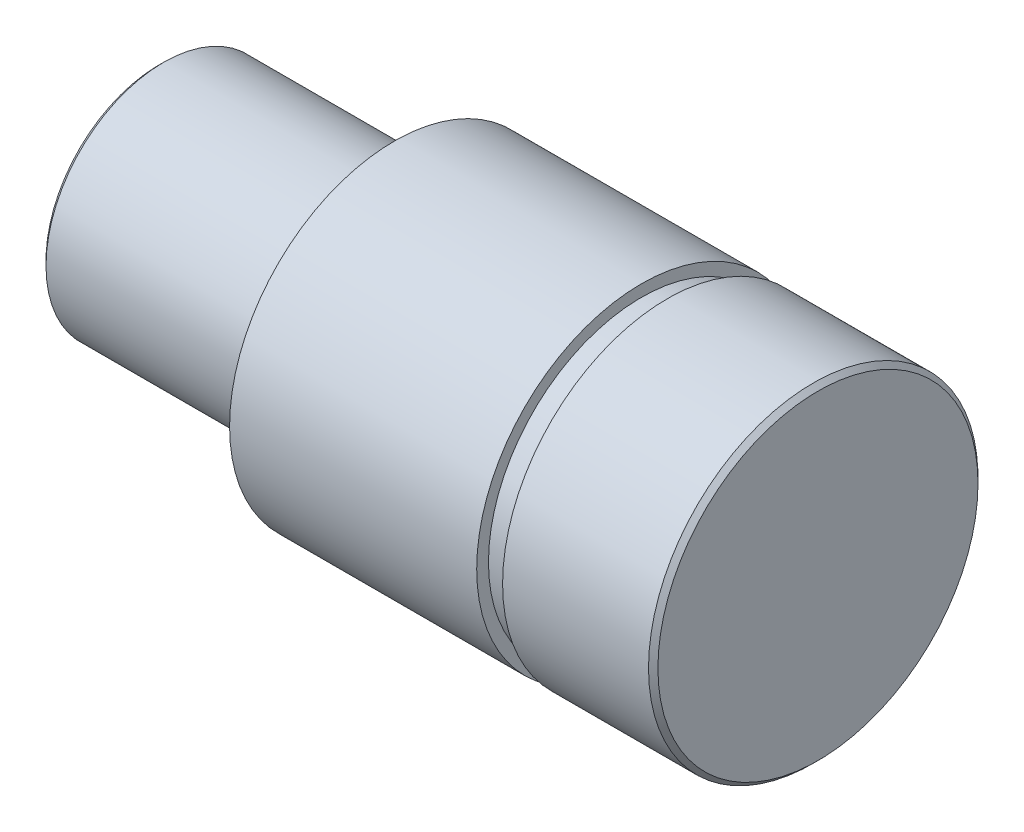
SolidWorks part; units mm, degrees
ref_plane "Front Plane" through (0, 0, 0) normal (0, 0, 1) x (1, 0, 0)
ref_plane "Top Plane" through (0, 0, 0) normal (0, 1, 0) x (1, 0, 0)
ref_plane "Right Plane" through (0, 0, 0) normal (1, 0, 0) x (0, 0, -1)
sketch "Sketch1" plane through (0, 0, 0) normal (0, 0, 1) x (1, 0, 0)
  line L0 (0, 0) -> (40.5225, 0) construction
  line L1 (0, 0) -> (0, 5)
  line L2 (0, 5) -> (10, 5)
  line L3 (10, 5) -> (10, 7)
  line L4 (10, 7) -> (28, 7)
  line L5 (28, 7) -> (28, 0)
  line L6 (28, 0) -> (0, 0)
  dimension "D1" = 10
  dimension "D2" = 14
  dimension "D3" = 18
  dimension "D4" = 10
revolve "Revolve1" add sketch "Sketch1" angle 360 about L0
chamfer "Chamfer1" distance 0.2 angle 45 1 edges at (0, 0, 5)
sketch "Sketch2" plane through (10, 0, 0) normal (-1, 0, 0) x (0, 0, 1)
  circle A0 centre (0, 0) radius 5 construction
  circle A1 centre (0, 0) radius 7
  circle A2 centre (0, 0) radius 7
  circle A3 centre (0, 0) radius 5
  dimension "D1" = 0
extrude "Cut-Extrude1" [suppressed] cut sketch "Sketch2" against normal blind 13
sketch "Sketch3" plane through (0, 0, 0) normal (0, 1, 0) x (1, 0, 0)
  line L0 (0, 0) -> (25, 0) construction
  line L1 (28, -7) -> (28, 7) construction
  circle A0 centre (25, 0) radius 1.5
  dimension "D1" = 3
  dimension "D2" = 3
extrude "Cut-Extrude2" [suppressed] cut sketch "Sketch3" against normal through all both and the other way through all
chamfer "Chamfer2" distance 0.2 angle 45 1 edges at (28, 0, 7)
sketch "Sketch4" plane through (0, 0, 0) normal (0, 1, 0) x (1, 0, 0)
  line L0 (0, 0) -> (25.4452, 0) construction
  line L1 (20.5, 8.8938) -> (21.6, 8.8938)
  line L2 (20.5, 8.8938) -> (20.5, 6.5)
  line L3 (20.5, 6.5) -> (21.6, 6.5)
  line L4 (21.6, 8.8938) -> (21.6, 6.5)
  line L5 (10, 7) -> (10, -7) construction
  dimension "D1" = 1.1
  dimension "D2" = 13
  dimension "D3" = 10.5
revolve "Cut-Revolve1" cut sketch "Sketch4" angle 360 about L0
